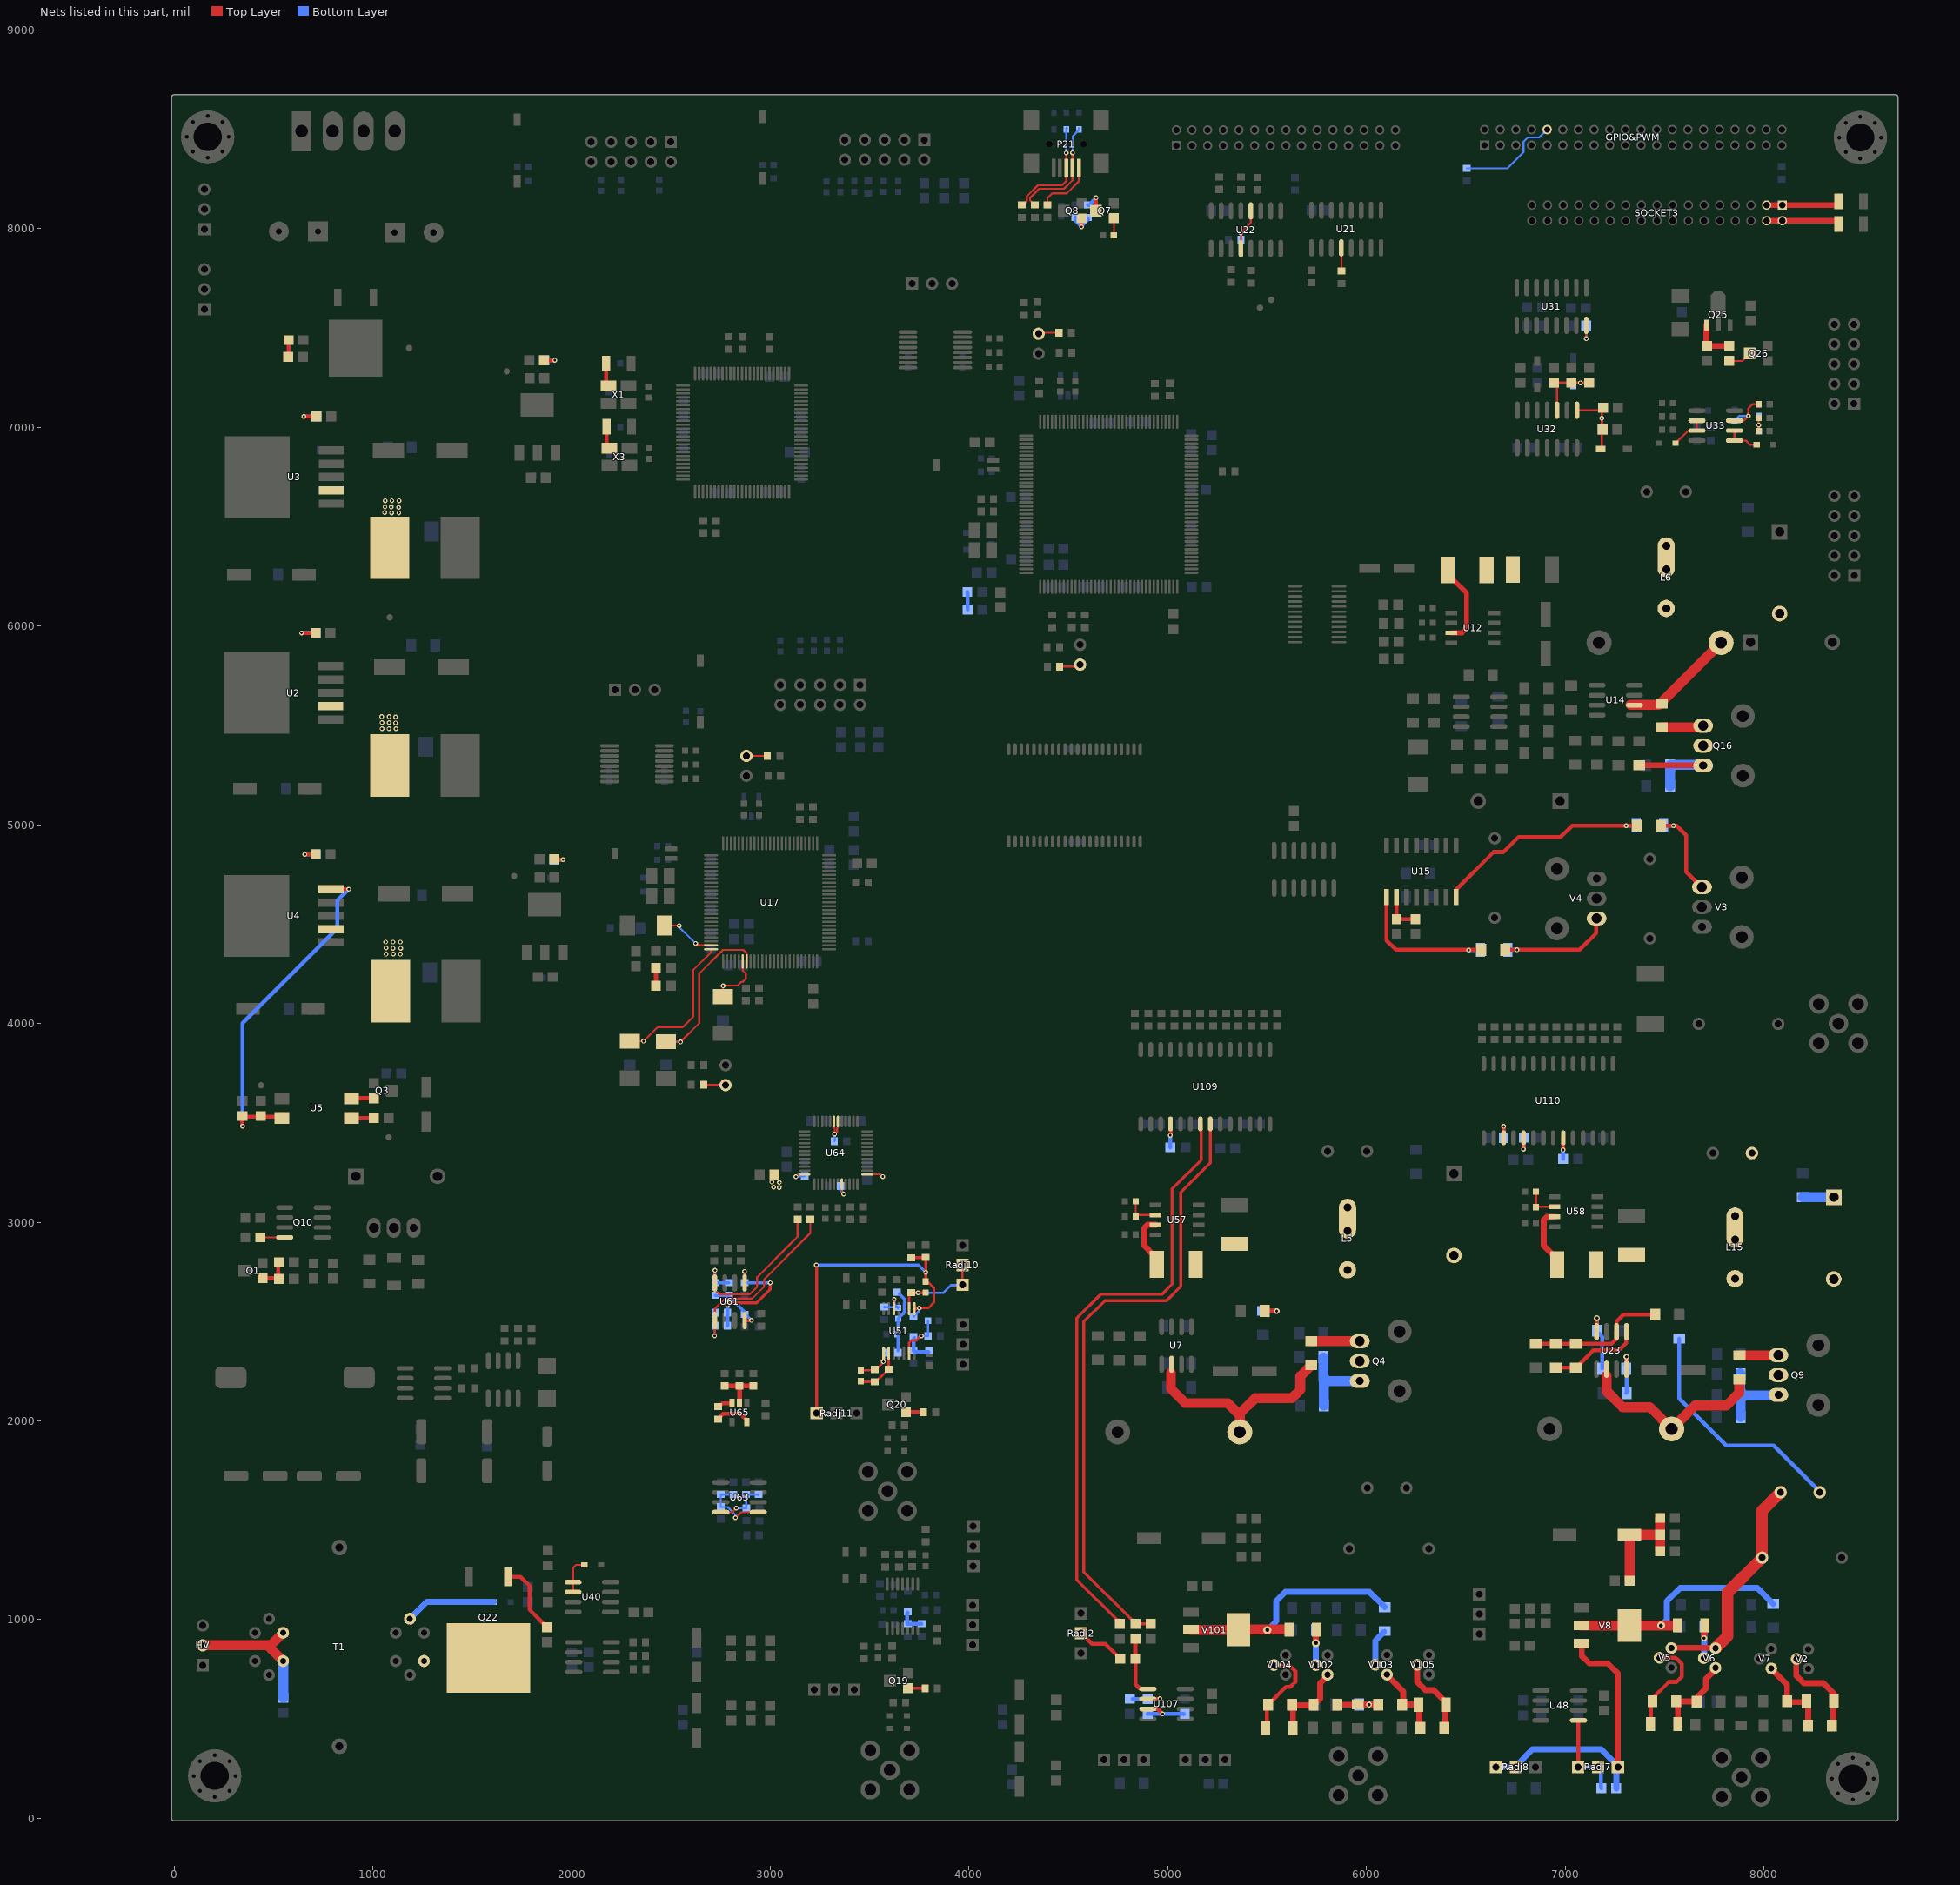
[diagram p0: the nets of this part, all layers, seen from the top]
# Altium PCB MISC82309.PcbDoc (part 10 of 14)
Units mil, origin at the board's own origin, x right, y up, seen from the top; angles counter-clockwise.
Board outline 8687.03 x 8687.86 mil, 4 copper layers (Top Layer, GND, POWER, Bottom Layer); 747 components, 583 nets, 2530 pads, 1834 vias.

## Via types
v1: diameter 24, hole 12, Top Layer to Bottom Layer, 1799 vias
v2: diameter 30, hole 15, Top Layer to Bottom Layer, 26 vias
v3: diameter 40, hole 20, Top Layer to Bottom Layer, 9 vias

## Nets (pads, with @x,y where several pads share a name; then routed paths per layer and width w, separated by ;. In a path a pad name is that pad's centre, name@x,y a point inside that pad or via, vN(x,y) a via of type N, cw(c..) or ccw(c..) an arc to the next point about the centre after c; other vN are vias at no path point) (continued)
NetC265_1: C265.1 R221.2 R227.1 R319.2 U23.2 | length 746.8
  Top Layer w15: R221.2@6852,2389 6854,2389 R221.2@6855,2389 ; U23.2@7258,2409 7258,2414 U23.2@7258,2449.49
  Top Layer w20: R221.2@6854,2388 6855,2389 6855.18,2389.18 7146.07,2389.18 7233.18,2389.18 U23.2@7257,2413 ; U23.2@7257,2449.49 U23.2@7257,2413 ; U23.2@7258,2414 U23.2@7257,2413 ; U23.2@7258,2449.49 7258,2500 7293,2535 R227.1@7445,2535
NetC265_2: C265.2 R319.1 U23.1 | length 465.8
  Top Layer w20: R319.1@6952,2269 7047,2269 7051,2265 C265.2@7054,2268 7111,2325 7111,2326 7140,2355 7270,2355 7307,2392 U23.1@7307,2448
NetC266_1: C266.1 D41.2 L16.1 R236.2 R313.2 | length 1343
  Bottom Layer w20: R236.2@7573,2414 7573,2113 7810,1876 8049,1876 L16.1@8276,1649
  Bottom Layer w50: R313.2@8196,3126 8340,3126 D41.2@8342,3124
NetC270_1: C270.1 R160.1 U23.8 | length 222.6
  Top Layer w20: U23.8@7308,2260.51 v2(7308,2323)
  Bottom Layer w20: R160.1@7305,2283 7308,2286 v2(7308,2323) ; C270.1@7307,2142 7309,2144 7309,2253 R160.1@7314,2258
NetC271_1: C271.1 R160.2 U23.4 | length 303.2
  Top Layer w20: U23.4@7158,2449.49 7158,2516 v2(7159,2517)
  Bottom Layer w20: C271.1@7157,2468 7159,2470 v2(7159,2517) ; C271.1@7169,2441 7187,2423 R160.2@7187,2263
NetC276_1: C276.1 Radj7.3 Radj8.1 Radj8.2 V8.3 | length 1519.1
  Top Layer w30: V8.3@7083,879.45 7083,819 7122,780 7214,780 7264,730 Radj7.3@7264,266
  Bottom Layer w30: Radj8.1@6651,259 6747,259 6835,347 7181,347 Radj7.3@7260,268 ; Radj7.3@7255,249 7256.5,247.5 C276.1@7256.5,151
NetC276_2: C276.2 Radj7.1 Radj7.2 U48.1 | length 426.7
  Top Layer w20: U48.1@7066.49,493 7066.49,278.51 Radj7.1@7070,275
  Bottom Layer w20: Radj7.1@7060,262 7063,259 Radj7.1@7065,259 Radj7.2@7165,259 ; Radj7.2@7179,251 7179,153.5 C276.2@7181.5,151
NetC277_1: C277.1 R291.2 R295.1 R296.2 TC3.2 | length 541.8
  Top Layer w30: R295.1@7466,1426 R295.1@7476.5,1415.5 ; C277.1@7476.5,1344 C277.1@7476.5,1350.5
  Top Layer w50: R291.2@7324.5,1195 TC3.2@7324.5,1420.5 ; TC3.2@7343,1427 R295.1@7476.5,1427 ; C277.1@7476.5,1350.5 R295.1@7476.5,1427 ; R296.2@7476.5,1512 R295.1@7476.5,1427
NetC279_2: C279.2 L16.2 R307.2 V5.3 V6.3 | length 1253.9
  Top Layer w30: V5.3@7534,857.21 7535.32,858.53 V6.3@7753.47,858.53
  Top Layer w60: V6.3@7759,860 7817,918 7817,1138 7989,1310 7989,1546.43 L16.2@8083.57,1641
  Bottom Layer w30: V6.3@7769,866 7816,913 R307.2@7816,965
NetC280_2: C280.2 R312.1 U57.2 | length 184.2
  Top Layer w10: R312.1@4839,3030 4839,3102 C280.2@4841,3104 ; R312.1@4843,3036 4844,3037 4876,3037 ; 4863,3037 4876,3037 ; U57.2@4939,3037 4876,3037
NetC281_2: C281.2 R344.1 U58.2 | length 174.9
  Top Layer w12: C281.2@6850,3156 6852.5,3153.5 R344.1@6852.5,3076 ; R344.1@6853,3076 6855,3078 U58.2@6946,3078
NetC282_2: C282.2 U110.19 | length 107.6
  Top Layer w20: v1(6789,3368) 6789,3423.99 U110.19@6790,3424.99
  Bottom Layer w20: v1(6789,3368) 6789,3414 C282.2@6792,3417
NetC284_1: C284.1 U110.17 | length 112.4
  Top Layer w20: U110.17@6690,3424.99 v1(6690,3482)
  Bottom Layer w20: C284.1@6689,3427 6690,3428 v1(6690,3482)
NetC285_2: C285.2 U110.23 | length 101.4
  Top Layer w20: v1(6989,3364) 6990,3365 U110.23@6990,3424.99
  Bottom Layer w20: v1@6987,3357 6989.5,3354.5 C285.2@6989.5,3318
NetC289_1: C289.1 R323.2 R324.1 U51.1 | length 185.7
  Top Layer w12: C289.1@3456,2255.5 3530.5,2255.5 3570,2295 v1@3570,2298 ; v1@3569,2295 v1(3569,2298)
  Bottom Layer w12: v1(3569,2298) 3569,2332.5 R324.1@3579.5,2343
NetC289_2: C289.2 R322.2 R323.1 U51.2 | length 246.8
  Top Layer w12: C289.2@3453,2197 3536,2197 3537,2198 3537,2202.5 R322.2@3595,2260.5 ; U51.2@3595.82,2340.8 3595.82,2265.18 R322.2@3596,2265
NetC290_1: C290.1 D48.1 R331.2 R332.2 Radj11.3 U51.8 | length 1784.9
  Top Layer w12: Radj11.3@3233,2039 Radj11.3@3233,2054 ; U51.8@3723.77,2565.2 3747.2,2565.2 v1(3750,2568) v1@3751.5,2569.5 ; v1@3752,2569 3796,2569 3824,2597 3824,2669 3793,2700 C290.1@3784,2700
  Top Layer w15: v1(3232,2785) 3234,2783 3234,2055 Radj11.3@3233,2054 ; R331.2@3710,2821.5 R332.2@3779.5,2821.5 ; C290.1@3780,2708 3782,2710 R332.2@3782,2819
  Bottom Layer w12: D48.1@3721,2525 3750,2554 v1@3750,2566
  Bottom Layer w15: v1(3232,2785) 3745,2785 v1(3782,2748)
NetC290_2: C290.2 R330.2 Radj10.2 Radj10.3 U51.9 | length 492.7
  Top Layer w12: U51.9@3698.18,2565.2 3698.18,2637.18 3707,2646 v1@3744,2646 ; v1(3744,2645) v1@3744,2646 ; C290.2@3786,2646 v1@3744,2646 ; Radj10.3@3959,2685 Radj10.3@3960,2684 ; Radj10.3@3967,2685 3967,2770 Radj10.2@3972,2775
  Bottom Layer w12: v1(3744,2645) 3871,2645 3909,2683 Radj10.3@3963,2683
NetC291_1: C291.1 R328.2 U51.12 | length 166
  Top Layer w12: U51.12@3621.41,2565.2 3621.41,2608.41 v1(3624,2611)
  Bottom Layer w12: R328.2@3574,2573.5 3574.5,2573 C291.1@3639.5,2573 ; v1@3625,2609 3625,2587.5 C291.1@3639.5,2573 ; C291.1@3643,2569.5 C291.1@3639.5,2573 ; C291.1@3646,2573 C291.1@3639.5,2573
NetC291_2: C291.2 C292.1 R324.2 R325.1 | length 312.6
  Bottom Layer w15: R324.2@3643,2353.5 C292.1@3643,2438 ; C292.1@3645,2439 3643,2441 C291.2@3643,2514.5 3676,2547.5 3676,2613 R325.1@3648,2641
NetC293_1: C293.1 R336.1 U51.6 | length 234.8
  Top Layer w12: U51.6@3698.18,2340.8 3698.18,2393.18 3710,2405 3733,2405 3756,2428 v1(3760,2428)
  Bottom Layer w12: v1(3760,2428) R336.1@3789,2428 ; R336.1@3793,2428 3793.5,2428.5 C293.1@3793.5,2505
NetC311_1: C311.1 R414.1 R415.1 U61.5 | length 956.9
  Top Layer w10: v1(2720,2428) 2721,2429 U61.5@2721,2505.51 ; U61.5@2721,2536 2721,2565 2772,2616 2909,2616 2968,2675 2968,2712 3202,2946 3202,3004.5 R415.1@3212,3014.5
  Bottom Layer w10: v1(2720,2428) 2720,2469 2719,2470 2719,2543 C311.1@2720,2544
NetC311_2: C311.2 R414.2 R417.1 U61.1 | length 633.1
  Top Layer w15: v1(2785,2584) v1@2787.5,2586.5 ; v1@2788,2586 2796.5,2594.5 2919.98,2594.5 2920.48,2594 2932,2594 3000,2662 v1(3000,2696) 3000,2698 v1@2999,2699 ; U61.1@2871,2694.49 v1(2871,2753)
  Bottom Layer w15: v1@2872,2754 R417.1@2872,2695.5 v1@2999.5,2695.5
  Bottom Layer w20: v1@2784.5,2583.5 C311.2@2784.5,2546 2785,2545.5 R414.2@2785,2480
NetC317_1: C317.1 C318.1 U15.2 | length 196
  Top Layer w20: C318.1@6151,4523 U15.2@6151,4636 ; C318.1@6152,4525.5 C317.1@6235,4525.5
NetC330_1: C330.1 R413.1 R416.2 U61.4 | length 880.6
  Top Layer w10: U61.4@2720,2660 U61.4@2722,2658 ; U61.4@2721,2694.49 2721,2757 v1(2722,2758) ; U61.4@2722,2669 U61.4@2722,2658 ; 3111,2901 3114,2904 ; R416.2@3137,3014.5 3137,2927 3114,2904 ; U61.4@2722,2658 2742,2638 2897,2638 2934,2675 2934,2724 3114,2904
  Bottom Layer w10: R413.1@2792,2695 R413.1@2793,2695
  Bottom Layer w15: v1@2723,2760 2721,2758 2721,2694 2722.5,2695.5 C330.1@2724,2695.5 R413.1@2792,2695.5
NetC330_2: C330.2 R412.1 R413.2 U61.8 | length 268.3
  Top Layer w15: U61.8@2871,2505.51 2904.51,2505.51 v1(2905,2506)
  Bottom Layer w15: C330.2@2724,2632.5 2786.5,2632.5 2853.5,2565.5 2871,2548 R412.1@2871,2543 ; R412.1@2871,2537.01 2874.99,2537.01 v1@2902,2510
  Bottom Layer w20: R413.2@2783.5,2632.5 R413.2@2787,2636
NetC363_1: C363.1 R373.1 R374.1 R375.2 | length 145.5
  Top Layer w10: R375.2@7972.5,6982 7972.5,7047 R373.1@7973.5,7048
  Bottom Layer w10: R374.1@7973,7057.5 v1(7973,7011) 7973,6980.5 C363.1@7974.5,6979
NetC364_2: C364.2 R372.1 U33.3 | length 256.6
  Top Layer w10: U33.3@7851.49,7034 7898,7034 v1(7921,7057) 7921,7095 7942,7116 R372.1@7973.5,7116
  Bottom Layer w10: C364.2@7852,7034.5 7874.5,7057 v1(7921,7057)
NetC373_2: C373.2 D54.2 R165.1 R491.2 R495.2 U32.3 | length 432.4
  Top Layer w10: C373.2@6943,7225.5 7119,7225.5 R491.2@7120,7224.5 ; U32.3@6959,7086.49 C373.2@6959,7209.5
  Bottom Layer w10: R495.2@6944,7224.5 v1(7076,7224.5)
NetC374_2: C374.2 D52.2 R493.2 R496.2 U32.1 | length 395.8
  Top Layer w10: U32.1@7059,7086.49 7193.01,7086.49 7184,7077.48 7184,6895.93 D52.2@7179.07,6891
  Bottom Layer w10: C374.2@7184,6985.49 v1(7184,7046)
NetC411_2: C411.2 C412.2 C413.2 L21.1 U64.8 U64.13 U64.30 U64.31 U64.48 | length 430.8
  Top Layer w10: L21.1@3021.5,3241 L21.1@3021.77,3240.73 ; v1(3129,3229) 3140.73,3240.73 U64.48@3172.52,3240.73 ; U64.31@3320.16,3506.48 3320.16,3475.78 3324,3471.94 v1(3324,3444) ; v1@3327,3446 3335.53,3454.53 3335.53,3472.41 3339.84,3476.73 U64.30@3339.84,3506.48 ; U64.8@3359.53,3191.52 3359.53,3154.47 3370,3144 v1(3370,3142) ; U64.13@3487.48,3240.73 3555.27,3240.73 v1(3566,3230)
  Bottom Layer w10: v1@3134,3230 3169.5,3230 C412.2@3173,3233.5 ; C411.2@3321.5,3408 3325,3411.5 v1@3325,3438
  Bottom Layer w15: C413.2@3353.5,3183 3353.5,3161.5 v1@3369,3146
  other v1: 3045,3174 3017,3177 3046,3200 3007,3202
NetC420_2: C420.2 C421.2 R479.1 U65.2 | length 230.4
  Top Layer w24: R479.1@2770,2176.5 C420.2@2845,2176.5 2845.5,2176.5 2846,2177 C421.2@2919,2177 ; C420.2@2844,2170 2845,2169 U65.2@2845,2089.24
NetC422_1: C422.1 U65.5 | length 163.9
  Top Layer w20: C422.1@2738,2009.5 2738,2012.78 2762.22,2037 2849,2037 U65.5@2877,2009
NetC422_2: C422.2 U65.3 | length 61.4
  Top Layer w20: C422.2@2750,2080 2759.24,2089.24 U65.3@2807.6,2089.24
NetC501_2: C501.2 R522.1 R523.2 U63.8 | length 256.9
  Top Layer w10: U63.8@2750.51,1541 2808,1541 v1@2826,1559
  Bottom Layer w10: v1(2829,1561) 2829.5,1561.5 R522.1@2879,1561.5 2879,1618 C501.2@2882,1621 ; C501.2@2878,1629.5 2937.5,1629.5 R523.2@2940,1627
NetC502_2: C502.2 R517.1 R524.2 U63.1 | length 352.3
  Top Layer w10: v1@2828,1516 2853,1541 U63.1@2939.49,1541
  Bottom Layer w10: R524.2@2750.51,1629.5 2750.51,1568.49 2752,1567 2786,1567 2824,1529 2824,1514 v1(2825,1513) ; R524.2@2751,1629 2751.5,1629.5 C502.2@2814,1629.5
NetD2_2: D2.2 L2.1 U2.2
  other v1: 1046,5484 1081,5484 1117,5484 1115,5513 1046,5514 1082,5514 1115,5543 1045,5544 1082,5544
NetD3_2: D3.2 L3.1 U3.2
  other v1: 1094,6570 1131,6570 1059,6571 1130,6598 1092,6599 1061,6600 1062,6631 1096,6631 1132,6631
NetD4_2: D4.2 L4.1 U4.2
  other v1: 1066,4349 1139,4349 1103,4350 1102,4379 1140,4379 1066,4380 1065,4410 1102,4410 1139,4410
NetD5_1: D5.1 L5.2 Q4.2
NetD6_2: D6.2 R23.1 U7.6 | length 1119.7
  Top Layer w20: U7.6@5019,2243 U7.6@5019,2285.51
  Top Layer w50: U7.6@5016,2243 5016,2162 5088,2090 5302,2090 5362.17,2029.83 ; D6.2@5362.17,1945 5362.17,2029.83 ; R23.1@5724,2282 5668,2226 5668,2158 5625,2115 5440,2115 5362.17,2037.17 5362.17,2029.83
NetD13_1: D13.1 L6.2 Q16.2
NetD14_2: D14.2 R81.1 U14.6 | length 586.2
  Top Layer w50: U14.6@7328,5603 7470.17,5603 D14.2@7784.17,5917
NetD23_2: D23.2 R106.2 U17.31 | length 331
  Top Layer w10: D23.2@2762,4135 v1(2762,4189) ; v1@2764,4187 2768,4191 2835.13,4191 2852.34,4208.21 2860.21,4208.21 2877,4225 2877,4251 2861.2,4266.8 U17.31@2861.2,4312.76
  Bottom Layer w10: R106.2@2762,4135 v1(2762,4189)
NetD27_2: D27.2 R197.2 R198.1 | length 130.4
  Bottom Layer w20: D27.2@3691,1035 3688,1032 3688,979 3688.5,979.5 R198.1@3691,979.5 R197.2@3761,979.5
NetD28_2: D28.2 R206.2 U17.24 | length 356.1
  Top Layer w10: D28.2@2466,4493 v1(2541,4493) ; v1(2624,4403) 2633.54,4393.46 U17.24@2701.76,4393.46
  Bottom Layer w10: R206.2@2466,4493 v1(2541,4493) 2541,4486 2607,4420 v1(2624,4403)
NetD29_2: D29.2 R207.2 U17.25 | length 823.8
  Top Layer w10: D29.2@2293,3911 D29.2@2295.5,3913.5 ; D29.2@2298,3911 v1(2362,3911) 2433,3982 2560,3982 2612,4034 2612,4269 2702,4359 U17.25@2702,4373 ; U17.25@2696,4373.78 U17.25@2701.76,4373.78
  Bottom Layer w10: R207.2@2292,3911 2361,3911 v1@2364,3908
NetD31_1: D31.1 U33.6 U33.7 | length 183.7
  Top Layer w10: D31.1@7555.32,6920 7619.32,6984 U33.7@7662.51,6984 U33.6@7662.51,7034
NetD32_1: D32.1 T1.4 | length 457.3
  Bottom Layer w30: T1.4@1186.33,1004.73 1270.6,1089 D32.1@1608.68,1089
NetD33_1: D33.1 U40.1 U40.2 | length 185.1
  Top Layer w10: U40.2@2007.51,1139 U40.1@2007.51,1189 2007.51,1260.51 2023,1276 D33.1@2064.68,1276
NetD34_2: D34.2 R110.2 U17.32 | length 869.1
  Top Layer w10: D34.2@2475,3909 v1@2549,3909 ; v1(2549,3907) 2551,3909 v1@2549,3909 ; U17.32@2880.89,4312.76 2880.89,4355.11 2865,4371 2762,4371 2642,4251 2642,4002 v1@2549,3909
  Bottom Layer w10: R110.2@2476,3911 2479,3908 v1@2547,3908
NetD35_2: D35.2 R98.1 U23.6 | length 1000.6
  Top Layer w20: U23.6@7208,2229 U23.6@7208,2260.51
  Top Layer w50: U23.6@7208,2229 7208,2150 7288,2070 7425.17,2070 D35.2@7535.17,1960 7652.17,2077 7811,2077 7876,2142 R98.1@7876,2210
NetD41_1: D41.1 L15.2 Q9.2
NetD42_1: D42.1 R310.1 V6.2 | length 206
  Top Layer w30: v2(7699,907) 7699,965.1 D42.1@7701.9,968
  Bottom Layer w30: R310.1@7700,966 7700,825 V6.2@7702,823
NetD42_2: D42.2 R297.2 V8.2 V8.4 | length 1222.3
  Top Layer w50: V8.2@7083,970 7339,970 V8.4@7339.55,970.55 ; V8.4@7323,970.55 V8.4@7339.55,970.55 ; V8.4@7341,972 V8.4@7339.55,970.55 ; D42.2@7555.55,970.55 V8.4@7339.55,970.55
  Bottom Layer w30: v3(7482,971) 7511,1000 7511,1093 7578,1160 7966,1160 8046,1080 R297.2@8046,1079
NetD43_1: D43.1 R300.2 V5.2 | length 500.5
  Top Layer w20: D43.1@7432,488 7432,597 7522,687 7561,687 7587,713 ; V5.2@7492,809 7555,809 7564,800 7587,777 7587,713 ; 7587.5,713.5 7587,713
  Top Layer w30: D43.1@7429.1,475 7435,480.9 D43.1@7435,488
NetD43_2: D43.2 R298.1 R300.1 V6.1 | length 416
  Top Layer w30: D43.2@7567,484 7567,581 R300.1@7559,589 7665,589 7666,588 7666,612 7708,654 7708,703 V6.1@7756,751
NetD44_1: D44.1 R299.2 R301.1 V7.1 | length 416.9
  Top Layer w30: V7.1@8038,751 8116,673 R299.2@8116,589 ; R299.2@8111,585 8211,585 8222,574 R301.1@8222,467
NetD44_2: D44.2 R301.2 V2.2 | length 454.8
  Top Layer w30: V2.2@8162,797 8162,720 8201,681 8298,681 8351.9,627.1 D44.2@8351.9,589 ; R301.2@8342,467 8350,475 D44.2@8350,575
NetD45_1: D45.1 R87.1 V3.1 | length 492.4
  Top Layer w20: R87.1@7482,4996 v1@7544,4996 ; v1(7544,4995) v1@7544,4996 ; V3.1@7685,4686 V3.1@7688,4686 ; V3.1@7685,4687 7609,4763 7609,4948 7561,4996 v1@7544,4996
  Bottom Layer w20: D45.1@7495,4995 v1(7544,4995)
NetD45_2: D45.2 R87.2 U15.8 | length 1120.1
  Top Layer w20: U15.8@6451,4636 6451,4674 6640,4863 6690,4863 6765,4938 6976,4938 6989,4951 ; 6989.5,4950.5 7035,4996 v1@7306,4996 ; v1(7306,4995) v1@7306,4996 ; R87.2@7354,4996 v1@7306,4996
  Bottom Layer w20: v1(7306,4995) D45.2@7351,4995
NetD48_2: D48.2 R333.2 R334.1 | length 132.1
  Bottom Layer w20: R333.2@3721,2353.5 3721,2412 D48.2@3726,2417 ; R333.2@3729,2347 R334.1@3795.5,2347
NetD49_1: D49.1 R92.1 V4.1 | length 600.4
  Top Layer w20: R92.1@6698,4371 v1(6757,4371) 6914,4371 7073,4371 7156,4454 V4.1@7156,4521
  Bottom Layer w20: D49.1@6716,4371 v1(6757,4371)
NetD49_2: D49.2 R92.2 U15.1 | length 757.5
  Top Layer w20: U15.1@6101,4636 6101,4418 6148,4371 v1@6514,4371 ; v1(6514,4370) v1@6514,4371 ; R92.2@6570,4371 v1@6514,4371
  Bottom Layer w20: v1(6514,4370) D49.2@6564,4370
NetD102_1: D102.1 R162.1 V102.2 | length 253.5
  Top Layer w30: v3(5745,882) 5745,946.1 D102.1@5748.9,950
  Bottom Layer w20: R162.1@5743,941 R162.1@5744.94,939.06 ; V102.2@5744.94,772 V102.2@5744.94,785.94
  Bottom Layer w30: V102.2@5740,781 V102.2@5744.94,785.94 ; R162.1@5744.94,939.06 V102.2@5744.94,785.94 ; V102.2@5745,786 V102.2@5744.94,785.94 ; R162.1@5745,941 R162.1@5745,948
NetD102_2: D102.2 R43.2 V101.2 V101.4 | length 1264.8
  Top Layer w50: V101.2@5116,949 V101.4@5310,949 ; V101.4@5316,950 D102.2@5611.1,950 ; V101.4@5340,949 V101.4@5350,959
  Bottom Layer w30: v3(5501,948) 5545,992 5545,1093 5592,1140 6015,1140 R43.2@6092,1063
NetD103_1: D103.1 R201.2 V104.2 | length 465.9
  Top Layer w20: D103.1@5492.1,455 5499,461.9 R201.2@5499,572 ; R201.2@5505,572 5594,661 5616,661 5642,687 5642,740 5612.68,769.32 5599,769.32 5547.68,769.32 5547,770 V104.2@5547,771
NetD103_2: D103.2 R40.1 R201.1 V102.1 | length 391.5
  Top Layer w30: D103.2@5629.9,455 5629.9,561.9 5637,569 5734,569 5767,602 5767,681 5803,717 V102.1@5804,717
NetD104_1: D104.1 R41.2 R42.1 V103.1 | length 369.7
  Top Layer w30: V103.1@6112,712 6185,639 6185,573 6266,573 6266,462 R42.1@6272,456
NetD104_2: D104.2 R42.2 V105.2 | length 404.3
  Top Layer w20: V105.2@6254.94,756 V105.2@6254.94,773 ; V105.2@6272,772 V105.2@6273.68,770.32
  Top Layer w30: V105.2@6255,756 6255,687 6296,646 6337,646 6397,586 6397,461 R42.2@6392,456
NetD131_1: D131.1 U33.1 U33.2 | length 169.9
  Top Layer w10: U33.2@7851.49,6984 U33.1@7851.49,6934 7909,6934 7930,6913 D131.1@7962.68,6913
NetD_BOOT0_1: D_BOOT0.1 R273.1 | length 105.5
  Top Layer w10: D_BOOT0.1@2880,5347 R273.1@2985.5,5347
NetD_BOOT1_1: D_BOOT1.1 R272.1 | length 109.9
  Top Layer w10: R272.1@2665.5,3691 2774,3691 D_BOOT1.1@2775,3690
NetESD24_1: ESD24.1 P21.2 R95.1 | length 570.1
  Top Layer w10: R95.1@4330,8119.5 4330,8120 4307,8143 4307,8154.96 4353.04,8201 4477.5,8201 4520.5,8244 P21.2@4520.5,8304.95 4520.5,8381.5 v1(4521,8382)
  Bottom Layer w10: v1(4521,8382) 4521,8465 4552,8496 ESD24.1@4552,8505.68
NetESD25_1: ESD25.1 P21.3 R96.1 | length 553.3
  Top Layer w10: R96.1@4266,8119.5 4269.5,8119.5 4290,8140 4290,8162 4346,8218 4468,8218 4489,8239 P21.3@4489,8304.95 v1(4489,8381)
  Bottom Layer w10: v1(4489,8381) 4489,8502.68 ESD25.1@4492,8505.68
NetFB1_2: FB1.2 X1.4 | length 119.8
  Top Layer w20: FB1.2@2174.01,7322 2174.01,7220.61 X1.4@2187,7207.61
NetFB4_2: FB4.2 X3.4 | length 113.6
  Top Layer w20: FB4.2@2176.01,7003 2176.01,6910.61 X3.4@2191,6895.61
NetFB18_1: FB18.1 U31.16 | length 132.8
  Top Layer w10: v1(7106,7446) U31.16@7106,7513.51
  Bottom Layer w10: FB18.1@7105.39,7511 7106,7510.39 v1(7106,7446)
NetFB25_2: FB25.2 SOCKET3.1 SOCKET3.3 | length 352.7
  Top Layer w30: SOCKET3.3@8013.26,8119 SOCKET3.1@8092,8119 8321,8119 FB25.2@8366,8119
NetFB26_2: FB26.2 SOCKET3.2 SOCKET3.4 | length 367.7
  Top Layer w30: SOCKET3.4@8013.26,8040.26 SOCKET3.2@8092,8040.26 8248,8040.26 8263.74,8040.26 8360.75,8040.26 FB26.2@8375.01,8026
NetFUSE1_1: FUSE1.1 U57.3 | length 216.3
  Top Layer w30: FUSE1.1@4927,2837 4882,2882 4882,2971 4898,2987 U57.3@4939,2987
NetFUSE1_2: FUSE1.2 FUSE14.2 L5.1 L5.3 | length 3.8
  Top Layer w50: FUSE1.2@5137,2829 FUSE1.2@5138,2828 ; FUSE14.2@5334,2880 5334,2881 FUSE14.2@5335,2882
NetFUSE2_1: FUSE2.1 U12.3 | length 356.9
  Top Layer w25: U12.3@6427,5966 6480,5966 6503,5989 6503,6167 FUSE2.1@6437,6233
NetFUSE2_2: FUSE2.2 FUSE13.2 L6.1 L6.3
NetFUSE12_1: FUSE12.1 U58.3 | length 250.9
  Top Layer w30: FUSE12.1@6935,2839 6892,2882 6892,3011 6909,3028 U58.3@6946,3028
NetFUSE12_2: FUSE12.2 FUSE15.2 L15.1 L15.3
NetGPIO&PWM_10: GPIO&PWM.10 R358.1 | length 516.3
  Bottom Layer w10: R358.1@6504,8303.5 6708.5,8303.5 6790,8385 6790,8437 6812,8459 6869.22,8459 GPIO&PWM.10@6908.96,8498.74
NetHV_2: HV.2 R293.1 T1.11 T1.12 | length 705.6
  Top Layer w50: HV.2@144,871 469.67,871 T1.11@548.54,792.13 ; 485.67,871 T1.12@548.54,933.87
  Bottom Layer w50: R293.1@550,607.5 T1.11@550,787
NetL11_1: L11.1 R277.2 | length 89.4
  Bottom Layer w20: L11.1@3991.5,6172 3992.5,6171 R277.2@3992.5,6083
NetL14_1: L14.1 R235.2 | length 90
  Top Layer w20: R235.2@2424.5,4190 L14.1@2424.5,4280
NetLED1_1: LED1.1 R1.2 | length 77.7
  Top Layer w20: LED1.1@1925,4828 1928,4825 v1(1957,4825)
  Bottom Layer w20: R1.2@1912.5,4825 v1(1957,4825)
NetLED2_1: LED2.1 R2.2 | length 139.3
  Top Layer w20: v1(641,5966) 642,5965 LED2.1@711.5,5965
  Bottom Layer w20: v1(641,5966) 708,5966 R2.2@709,5965
NetLED3_1: LED3.1 R3.2 | length 117.5
  Top Layer w20: v1(653,7055) LED3.1@707,7055
  Bottom Layer w20: v1(653,7055) R3.2@716.5,7055
NetLED4_2: LED4.2 R4.2 | length 111.9
  Top Layer w20: v1(658,4851) LED4.2@715.5,4851
  Bottom Layer w20: v1(658,4851) 711,4851 R4.2@712,4850
NetLED5_1: LED5.1 R9.1 | length 85.2
  Top Layer w20: LED5.1@575,7354 575.5,7354.5 R9.1@575.5,7439
NetLED6_1: LED6.1 R16.2 | length 107
  Top Layer w20: LED6.1@1861.5,7338 v1(1916,7338)
  Bottom Layer w20: R16.2@1863.5,7338 v1(1916,7338)
NetP21_1: P21.1 R57.1 | length 294.2
  Top Layer w10: R57.1@4394,8119.5 4394,8154 4418,8178 4492,8178 4551.99,8237.99 P21.1@4551.99,8304.95
NetP_BOOT0_1: P_BOOT0.1 R271.1 | length 109.9
  Top Layer w10: P_BOOT0.1@4351,7475 4352,7476 R271.1@4460.5,7476
NetP_BOOT1_1: P_BOOT1.1 R270.1 | length 102.5
  Top Layer w10: R270.1@4456.5,5796 P_BOOT1.1@4559,5796
NetQ1_1: Q1.1 R12.2 R13.1 | length 161.2
  Top Layer w20: Q1.1@444,2718 523.5,2718 523.5,2794 R13.1@527.5,2798
NetQ3_2: Q3.2 U5.2 | length 109.6
  Top Layer w20: U5.2@893.2,3624.2 Q3.2@1002.8,3624.2
NetQ4_1: Q4.1 R23.2 | length 252
  Top Layer w50: R23.2@5722,2402 Q4.1@5974,2402
NetQ4_3: Q4.3 R25.2 R28.2 R29.2 | length 420.9
  Bottom Layer w50: R25.2@5784,2318 5784,2205 5789,2200 5790,2201 Q4.3@5966,2201 ; R29.2@5785,2201 5785,2079 R28.2@5786,2078
NetQ7_1: Q7.1 R149.2 | length 86.7
  Top Layer w10: R149.2@4728.5,7966 4729,7966.5 Q7.1@4729,8052.5
NetQ7_3: Q7.3 R226.2 | length 114.5
  Top Layer w20: Q7.3@4639,8090.5 v1(4639,8155)
  Bottom Layer w20: R226.2@4599,8119.5 4604.5,8119.5 v1@4636,8151
NetQ8_1: Q8.1 R150.1 R226.1 | length 147.6
  Top Layer w20: v1(4566,8009) Q8.1@4566,8052
  Bottom Layer w20: R150.1@4535,8056.5 4535,8042 4564,8013 4598,8047 R226.1@4599,8047
NetQ9_1: Q9.1 R98.2 | length 213.3
  Top Layer w20: Q9.1@8050,2330 Q9.1@8056,2336
  Top Layer w50: R98.2@7877,2330 8079,2330 Q9.1@8081,2328
NetQ9_3: Q9.3 R157.2 R158.2 R159.2 | length 425.1
  Bottom Layer w50: R159.2@7881,2240 7881,2121 7882,2120 R157.2@7882,2020 ; R158.2@7882,2129 8081,2129 Q9.3@8085,2133
NetQ10_4: Q10.4 R399.1 | length 123
  Top Layer w10: R399.1@433.5,2924 Q10.4@556.51,2924
NetQ16_1: Q16.1 R81.2 | length 218.8
  Top Layer w50: R81.2@7486,5490 7685,5490 Q16.1@7699,5504
NetQ16_3: Q16.3 R82.2 R84.2 R85.2 | length 590.3
  Top Layer w30: R82.2@7372,5300 Q16.3@7681,5300
  Bottom Layer w30: R85.2@7527,5285 R85.2@7542,5300
  Bottom Layer w50: R84.2@7527,5195 7527,5297 7532,5302 Q16.3@7683,5302
NetQ19_1: Q19.1 R378.1 | length 80.2
  Top Layer w15: Q19.1@3692,654.5 3760.5,654.5 3761,655 R378.1@3772,655
NetQ20_1: Q20.1 R379.1 | length 82.2
  Top Layer w20: Q20.1@3683,2044.5 3764.5,2044.5 R379.1@3765,2044
NetQ22_1: Q22.1 R215.1 | length 370.7
  Top Layer w20: Q22.1@1682,1215.72 1743,1215.72 1788,1170.72 1788,1050.5 R215.1@1877,961.5
NetQ22_2: Q22.2 T1.1
NetQ25_1: Q25.1 R283.1 R284.2 | length 223.1
  Top Layer w30: Q25.1@7710.94,7515.13 7711,7515.08 7711,7409.5 7827,7409.5 R284.2@7828,7410.5
NetQ26_3: Q26.3 R284.1 | length 118.5
  Top Layer w10: R284.1@7825,7334.5 7890.5,7334.5 Q26.3@7928,7372
NetR5_2: R5.2 U5.1 | length 111.6
  Top Layer w20: U5.1@893.2,3523.8 R5.2@1004.8,3523.8
NetR6_1: R6.1 R11.2 U4.5 U5.4 | length 1747.6
  Top Layer w20: v1(345,3483) R6.1@345,3534.5 348.5,3531 R11.2@439,3531 ; R11.2@449,3532 534.61,3532 U5.4@542.8,3523.8 ; U4.5@789.22,4675.86 v1(878.86,4675.86)
  Bottom Layer w20: v1(345,3483) 345,4002 822,4479 822,4620 v1@878,4676
NetR18_2: R18.2 R19.1 | length 123.2
  Top Layer w20: R18.2@5487,2554 5547,2554 v2(5548,2553)
  Bottom Layer w20: R19.1@5481,2554 v2@5540,2554 ; v2@5552,2552 v2@5554,2554
NetR22_1: R22.1 U109.21 | length 3055.7
  Top Layer w10: R22.1@4759,978.5 R22.1@4759,998
  Top Layer w15: R22.1@4759,998 4745,998 4543,1200 4543,2518 4662,2637 4971,2637 5022,2688 5022,3167 5168,3313 5168,3490.99 U109.21@5164,3494.99
NetR27_2: R27.2 R31.1 U107.6 | length 199.1
  Top Layer w20: U107.6@4899.51,601 4959,601 v1(4960,602)
  Bottom Layer w20: R27.2@4823,601 4824,600 4958,600 v1(4960,602)
NetR30_1: R30.1 R33.2 U109.22 | length 3111.3
  Top Layer w10: U109.22@5214,3481 U109.22@5214,3494.99
  Top Layer w15: R30.1@4822,996 4578,1240 4578,2500 4684,2606 4994,2606 5066,2678 5066,3151 5214,3299 U109.22@5214,3481 ; R30.1@4848,978 4848.5,978.5 R33.2@4914,978.5
NetR30_2: R30.2 R32.2 U107.5 | length 292
  Top Layer w20: R32.2@4836.5,803 R30.2@4836.5,902.5 ; R32.2@4837,795 4837,675 4861,651 U107.5@4899.51,651
NetR31_2: R31.2 R47.1 U107.7 | length 267.1
  Top Layer w20: U107.7@4899.51,551 4949,551 v1(4974,526)
  Bottom Layer w20: R31.2@4899,525.5 5080.5,525.5 R47.1@5081,525
NetR32_1: R32.1 Radj2.2 | length 228.7
  Top Layer w20: Radj2.2@4580,917 4618,879 4685.5,879 R32.1@4761.5,803
NetR34_1: R34.1 U109.18 | length 115.6
  Top Layer w20: v1(5013,3438) 5014,3439 U109.18@5014,3494.99
  Bottom Layer w20: v1@5013,3435 5013.5,3434.5 R34.1@5013.5,3377
NetR35_1: R35.1 U21.4 | length 103.4
  Top Layer w10: U21.4@5873,7903.51 5874,7902.51 R35.1@5874,7800.5
NetR36_1: R36.1 U22.4 U22.12 | length 243.9
  Top Layer w10: U22.4@5368,7900.51 v1(5368,7979) 5368,7980 5418,8030 U22.12@5418,8089.49
  Bottom Layer w10: R36.1@5367.5,7945 5368,7945.5 v1(5368,7979)
NetR40_2: R40.2 R41.1 R164.1 R202.1 | length 259.8
  Top Layer w30: R40.2@5854,572 5947,572 5948,573 6061,573 R41.1@6062,572
  Bottom Layer w30: R164.1@5962,573 v2(6013,573)
NetR43_1: R43.1 V103.2 | length 189.6
  Bottom Layer w20: R43.1@6085.5,936.5 R43.1@6092,943
  Bottom Layer w30: V103.2@6043.94,773 6043.94,893.94 R43.1@6086,936